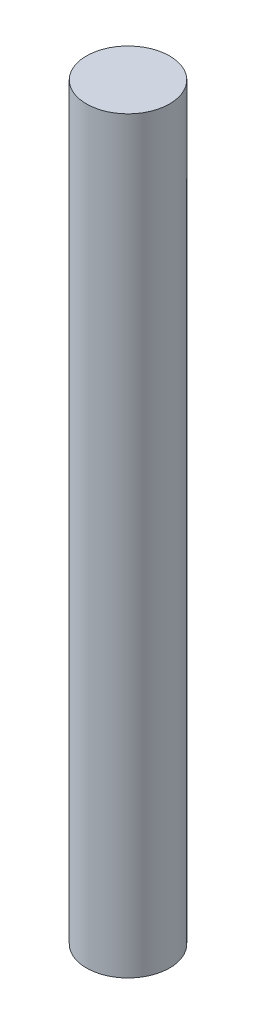
from build123d import *

# Parameters (mm, degrees)
SKETCH1_R           = 10
BOSS_EXTRUDE1_DEPTH = 180


with BuildPart() as part:
    # Sketch1 → Boss-Extrude1 (new body)
    with BuildSketch(Plane(origin=(0, 0, 0), x_dir=(1, 0, 0), z_dir=(0, 1, 0))):
        with Locations(Location((0, 0, 0), (0, 0, 90))):
            Circle(SKETCH1_R)
    extrude(amount=BOSS_EXTRUDE1_DEPTH)


solid = part.part
